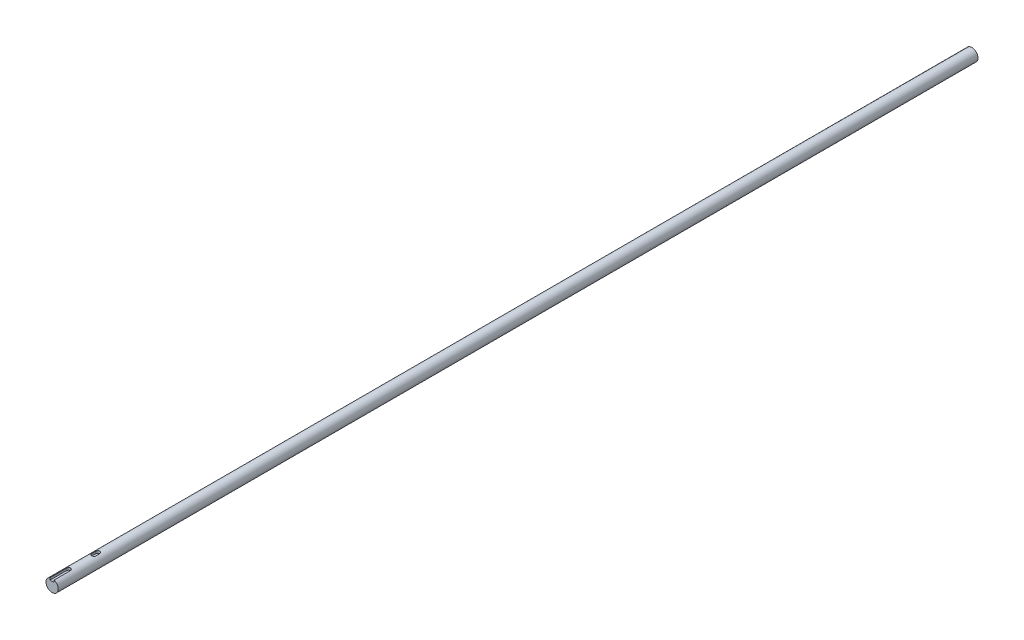
SolidWorks part; units mm, degrees
ref_plane "前视基准面" through (0, 0, 0) normal (0, 0, 1) x (1, 0, 0)
ref_plane "上视基准面" through (0, 0, 0) normal (0, 1, 0) x (1, 0, 0)
ref_plane "右视基准面" through (0, 0, 0) normal (1, 0, 0) x (0, 0, -1)
sketch "草图1" plane through (0, 0, 0) normal (0, 0, 1) x (1, 0, 0)
  circle A0 centre (0, 0) radius 7.5
  dimension "D1" = 15
extrude "凸台-拉伸1" add sketch "草图1" along normal blind 1130
sketch "草图2" plane through (0, 0, 1130) normal (0, 0, 1) x (1, 0, 0)
  line L0 (0, 0) -> (0, 7.5) construction
  line L1 (-2.5, 7.0711) -> (-2.5, 4.5)
  line L2 (2.5, 7.0711) -> (2.5, 4.5)
  line L3 (-2.5, 4.5) -> (2.5, 4.5)
  circle A0 centre (0, 0) radius 7.5 construction
  circle A1 centre (0, 0) radius 7.5 construction
  arc A2 (-2.5, 7.0711) -> (2.5, 7.0711) centre (0, 0) cw
  dimension "D1" = 2.5
  dimension "D2" = 3
extrude "切除-拉伸1" cut sketch "草图2" against normal blind 20
sketch "草图3" plane through (0, 4.5, 0) normal (0, 1, 0) x (1, 0, 0)
  line L0 (-2.5, -1110) -> (2.5, -1110) construction
  line L1 (-2.5, -1110) -> (2.5, -1110)
  arc A0 (-2.5, -1110) -> (2.5, -1110) centre (0, -1110) cw
extrude "切除-拉伸2" cut sketch "草图3" along normal up to next
ref_plane "基准面1" through (0, 4.5, 0) normal (0, 1, 0) x (1, 0, 0)
sketch "草图5" plane through (0, 4.5, 0) normal (0, 1, 0) x (1, 0, 0)
  line L0 (0, -1079.079) -> (0, -1074.079) construction
  line L1 (0, -8.25) -> (0, 8.25) construction
  line L2 (-2.5, -1079.079) -> (-2.5, -1074.079)
  line L3 (2.5, -1079.079) -> (2.5, -1074.079)
  arc A0 (-2.5, -1079.079) -> (2.5, -1079.079) centre (0, -1079.079) ccw
  arc A1 (2.5, -1074.079) -> (-2.5, -1074.079) centre (0, -1074.079) ccw
  point P5 (0, -1076.579)
  dimension "D1" = 5
  dimension "D2" = 10
extrude "切除-拉伸3" cut sketch "草图5" along normal blind 17
